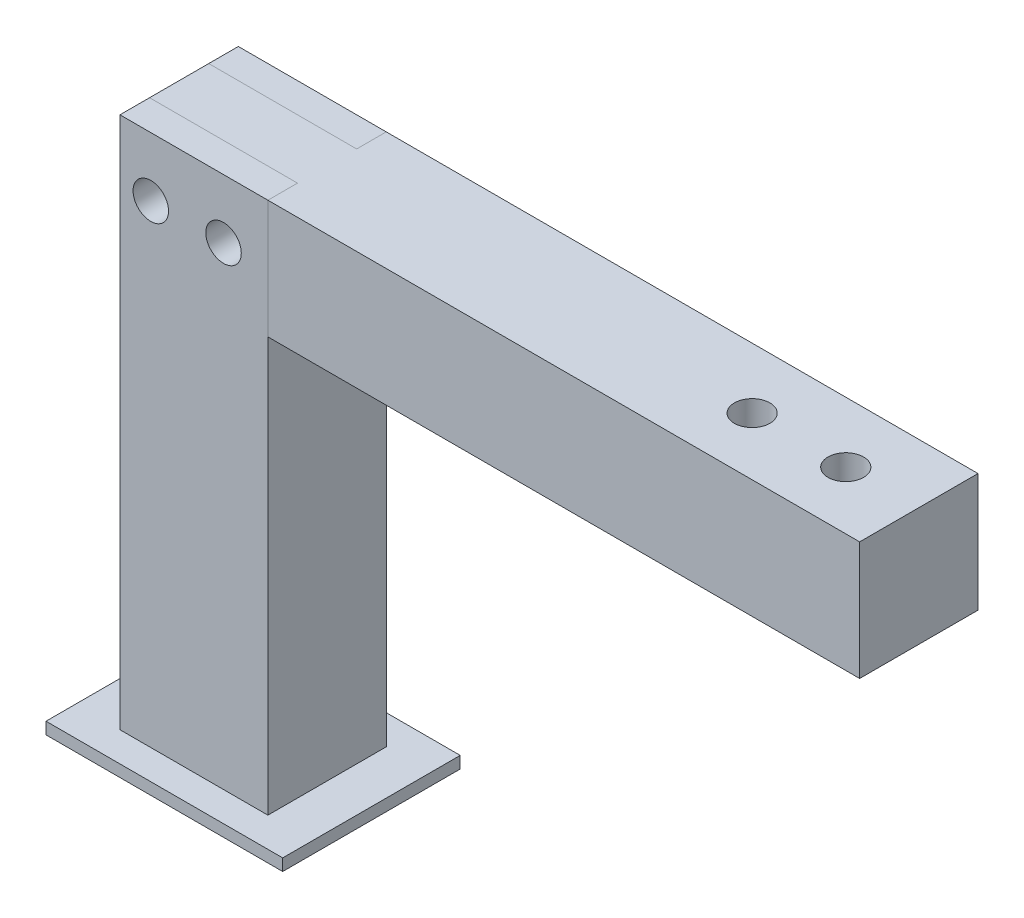
SolidWorks part; units mm, degrees
ref_plane "Front Plane" through (0, 0, 0) normal (0, 0, 1) x (1, 0, 0)
ref_plane "Top Plane" through (0, 0, 0) normal (0, 1, 0) x (1, 0, 0)
ref_plane "Right Plane" through (0, 0, 0) normal (1, 0, 0) x (0, 0, -1)
other "Configuration Table"
sketch "Sketch1" plane through (0, 0, 0) normal (0, 1, 0) x (1, 0, 0)
  line L0 (-35, 0.2436) -> (25, 0.2436) construction
  line L5 (-35, 77.7436) -> (-35, -77.2564) construction
  line L6 (25, -77.2564) -> (25, 77.7436) construction
  line L8 (-25, 15.2436) -> (15, 15.2436)
  line L9 (-25, 15.2436) -> (-25, -14.7564)
  line L10 (-25, -14.7564) -> (15, -14.7564)
  line L11 (15, 15.2436) -> (15, -14.7564)
  line L12 (-25, 15.2436) -> (15, -14.7564) construction
  line L13 (-25, -14.7564) -> (15, 15.2436) construction
  point P6 (-5, 0.2436)
extrude "Boss-Extrude1" add sketch "Sketch1" along normal blind 2
sketch "Sketch5" plane through (0, 2, 0) normal (0, 1, 0) x (1, 0, 0)
  line L1 (-17.5, 10.2436) -> (7.5, 10.2436)
  line L2 (-17.5, 10.2436) -> (-17.5, -9.7564)
  line L3 (-17.5, -9.7564) -> (7.5, -9.7564)
  line L4 (7.5, 10.2436) -> (7.5, -9.7564)
  line L5 (-17.5, 10.2436) -> (7.5, -9.7564) construction
  line L6 (-17.5, -9.7564) -> (7.5, 10.2436) construction
  point P0 (-5, 0.2436)
extrude "Boss-Extrude2" add sketch "Sketch5" along normal blind 90
sketch "Sketch6" plane through (0, 92, 0) normal (0, 1, 0) x (1, 0, 0)
  line L0 (7.5, -9.7564) -> (7.5, 10.2436) construction
  line L1 (-17.5, 5.2436) -> (7.5, 5.2436)
  line L2 (-17.5, 5.2436) -> (-17.5, -4.7564)
  line L3 (-17.5, -4.7564) -> (7.5, -4.7564)
  line L4 (7.5, 5.2436) -> (7.5, -4.7564)
  line L5 (-17.5, 5.2436) -> (7.5, -4.7564) construction
  line L6 (-17.5, -4.7564) -> (7.5, 5.2436) construction
  point P0 (-5, 0.2436)
extrude "Cut-Extrude3" cut sketch "Sketch6" against normal blind 20
sketch "Sketch7" plane through (0, 72, 0) normal (0, 1, 0) x (1, 0, 0)
  line L0 (7.5, -4.7564) -> (7.5, -9.7564)
  line L1 (-17.5, 5.2436) -> (7.5, 5.2436)
  line L2 (-17.5, 5.2436) -> (-17.5, -4.7564)
  line L3 (-17.5, -4.7564) -> (7.5, -4.7564)
  line L5 (7.5, 10.2436) -> (107.5, 10.2436)
  line L6 (7.5, 10.2436) -> (7.5, 5.2436)
  line L7 (7.5, -9.7564) -> (107.5, -9.7564)
  line L8 (107.5, 10.2436) -> (107.5, -9.7564)
extrude "Boss-Extrude3" add sketch "Sketch7" along normal blind 20 separate body
sketch "Sketch8" plane through (0, 92, 0) normal (0, 1, 0) x (1, 0, 0)
  circle A0 centre (95.3981, 0) radius 3
  circle A1 centre (79.5745, 0) radius 3
extrude "Cut-Extrude4" cut sketch "Sketch8" against normal blind 20
sketch "Sketch9" plane through (0, 0, 9.7564) normal (0, 0, 1) x (1, 0, 0)
  circle A0 centre (-12.29, 82) radius 3
  circle A1 centre (0, 82) radius 3
extrude "Cut-Extrude5" cut sketch "Sketch9" against normal blind 29
